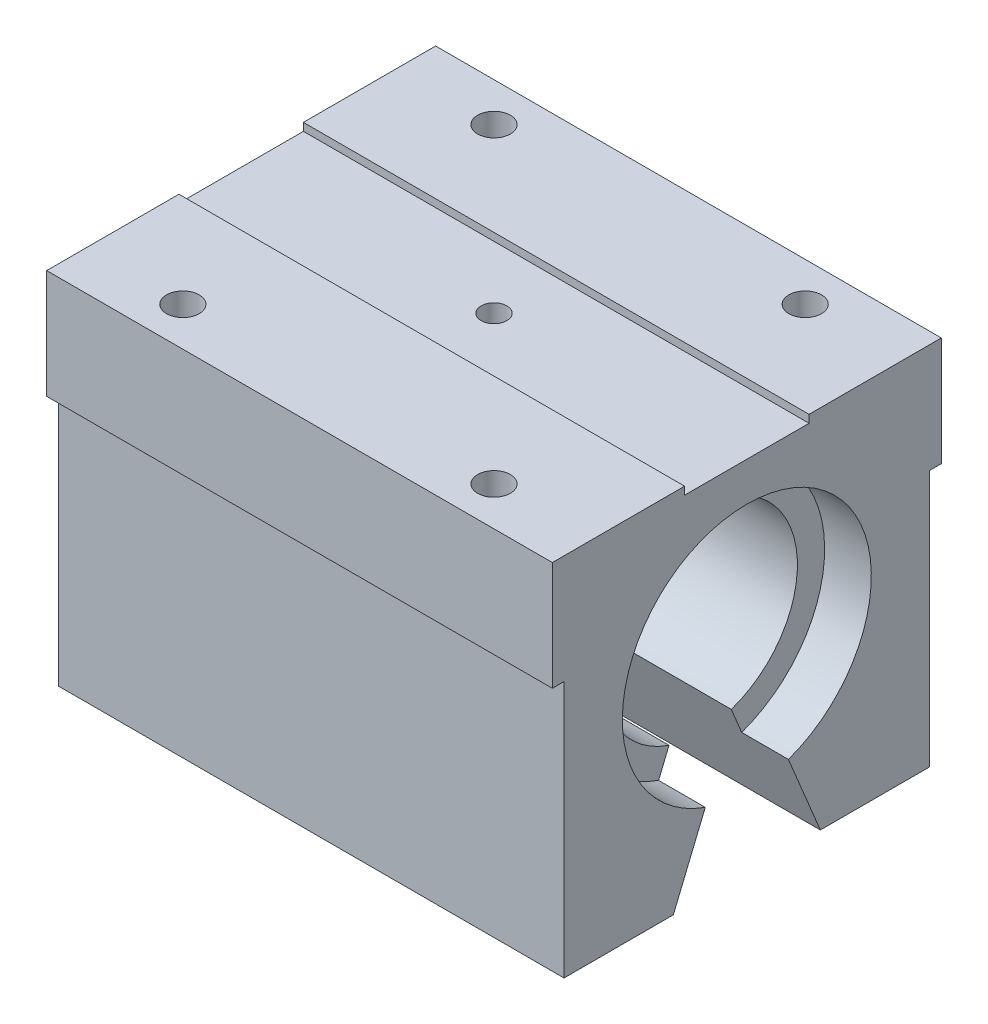
from build123d import *

# Parameters (mm, degrees)
EXTRUDE1_DEPTH            = 65
SKETCH2_R                 = 16
EXTRUDE2_DEPTH            = 6
EXTRUDE3_START            = -6
SKETCH3_R                 = 16
EXTRUDE3_DEPTH            = 6
M5X0_8_TAPPED_HOLE1_D     = 4.2
M5X0_8_TAPPED_HOLE1_DEPTH = 12.4
M5X0_8_TAPPED_HOLE1_TIP   = 1.2618073
M4X0_7_TAPPED_HOLE1_D     = 3.3
M4X0_7_TAPPED_HOLE1_DEPTH = 10.1
M4X0_7_TAPPED_HOLE1_TIP   = 0.991420021


with BuildPart() as part:
    # Sketch1 → Extrude1 (new body)
    with BuildSketch(Plane(origin=(0, 0, 0), x_dir=(0, 0, -1), z_dir=(1, 0, 0))):
        with BuildLine():
            Line((-23.5, -25), (-9.449924117, -25))
            Line((-9.449924117, -25), (-4, -11.842719282))
            ThreePointArc((-4, -11.842719282), (0, 12.5), (4, -11.842719282))
            Line((4, -11.842719282), (9.449924117, -25))
            Line((9.449924117, -25), (23.5, -25))
            Line((23.5, -25), (23.5, 8))
            Line((23.5, 8), (25, 8))
            Line((25, 8), (25, 22))
            Line((25, 22), (8, 22))
            Line((8, 22), (8, 21))
            Line((8, 21), (-8, 21))
            Line((-8, 21), (-8, 22))
            Line((-8, 22), (-25, 22))
            Line((-25, 22), (-25, 8))
            Line((-25, 8), (-23.5, 8))
            Line((-23.5, 8), (-23.5, -25))
        make_face()
    extrude(amount=EXTRUDE1_DEPTH)

    # Sketch2 → Extrude2 (cut)
    with BuildSketch(Plane(origin=(65, 0, 0), x_dir=(0, 0, -1), z_dir=(1, 0, 0))):
        Circle(SKETCH2_R)
    extrude(amount=-EXTRUDE2_DEPTH, mode=Mode.SUBTRACT)

    # Sketch3 → Extrude3 (cut)
    with BuildSketch(Plane.ZY.offset(EXTRUDE3_START)):
        Circle(SKETCH3_R)
    extrude(amount=EXTRUDE3_DEPTH, mode=Mode.SUBTRACT)

    # M5x0.8 Tapped Hole1
    with Locations(Plane(origin=(12.5, 22, -20), x_dir=(0, 0, 1), z_dir=(0, 1, 0))):
        with Locations((0, 0), (0, 40), (40, 0), (40, 40)):
            Hole(M5X0_8_TAPPED_HOLE1_D / 2, depth=M5X0_8_TAPPED_HOLE1_DEPTH)
            with Locations((0, 0, -(M5X0_8_TAPPED_HOLE1_DEPTH + M5X0_8_TAPPED_HOLE1_TIP / 2))):  # 118° drill point
                Cone(0, M5X0_8_TAPPED_HOLE1_D / 2, M5X0_8_TAPPED_HOLE1_TIP, mode=Mode.SUBTRACT)

    # M4x0.7 Tapped Hole1
    with Locations(Plane(origin=(32.5, 22, 0), x_dir=(0, 0, 1), z_dir=(0, 1, 0))):
        with Locations((0, 0)):
            Hole(M4X0_7_TAPPED_HOLE1_D / 2, depth=M4X0_7_TAPPED_HOLE1_DEPTH)
            with Locations((0, 0, -(M4X0_7_TAPPED_HOLE1_DEPTH + M4X0_7_TAPPED_HOLE1_TIP / 2))):  # 118° drill point
                Cone(0, M4X0_7_TAPPED_HOLE1_D / 2, M4X0_7_TAPPED_HOLE1_TIP, mode=Mode.SUBTRACT)


solid = part.part
